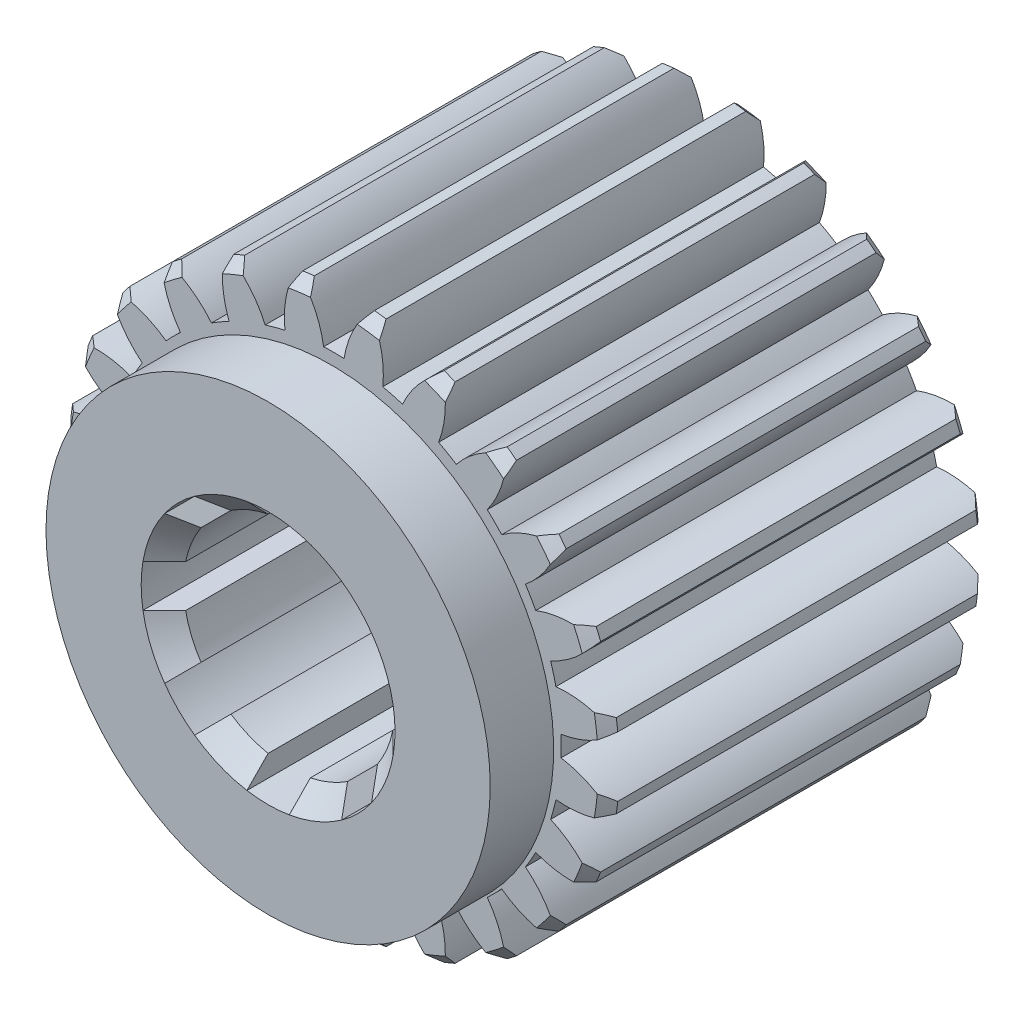
from build123d import *

# Parameters (mm, degrees)
BOSS_EXTRUDE1_DEPTH = 18
SKETCH2_R           = 10.5
BOSS_EXTRUDE2_DEPTH = 3
CUT_EXTRUDE1_DEPTH  = 43.00000000000001
CHAMFER1_SIZE       = 1
CHAMFER2_SIZE       = 0.5
CHAMFER3_SIZE       = 0.5


with BuildPart() as part:
    # Sketch1 → Boss-Extrude1 (new body)
    with BuildSketch(Plane.XY):
        with BuildLine():
            ThreePointArc((-12.813792243846223, 1.7470560088445317), (-11.780957931307613, 1.140113023790045), (-10.629995743569133, 0.8078291893048202))
            ThreePointArc((-10.629995743569133, 0.8078291893048202), (-10.640873065015485, 0.3243808049535287), (-10.629995743569129, -0.15906757939776273))
            ThreePointArc((-10.629995743569129, -0.15906757939776273), (-11.780957931307606, -0.49135141388299797), (-12.813792243846212, -1.0982943989374916))
            ThreePointArc((-12.813792243846212, -1.0982943989374916), (-12.780656262875008, -1.3724596939071496), (-12.741703962830215, -1.6458592559440115))
            ThreePointArc((-12.741703962830215, -1.6458592559440115), (-11.586974222248184, -1.9648039697727557), (-10.389228735284952, -1.9878745727808178))
            ThreePointArc((-10.389228735284952, -1.9878745727808178), (-10.274609771796674, -2.4576651108534753), (-10.13897743689663, -2.9218251330260894))
            ThreePointArc((-10.13897743689663, -2.9218251330260894), (-11.164720154370919, -3.5406776047933204), (-12.005273087305993, -4.3942566996627965))
            ThreePointArc((-12.005273087305993, -4.3942566996627965), (-11.902306987662186, -4.650503815792648), (-11.793920941477731, -4.9045059165580325))
            ThreePointArc((-11.793920941477731, -4.9045059165580325), (-10.595988696391819, -4.91371680399467), (-9.433084285772368, -4.626001952056541))
            ThreePointArc((-9.433084285772368, -4.626001952056541), (-9.200780130294392, -5.050119195046481), (-8.949635901421074, -5.463359116590063))
            ThreePointArc((-8.949635901421074, -5.463359116590063), (-9.78025647755529, -6.326606452390418), (-10.371245737586712, -7.36865165236567))
            ThreePointArc((-10.371245737586712, -7.36865165236567), (-10.2054664888015, -7.589517772159847), (-10.035033026408444, -7.806812588244913))
            ThreePointArc((-10.035033026408444, -7.806812588244913), (-8.875535379644617, -7.505661942532346), (-7.826722059162263, -6.926768927336334))
            ThreePointArc((-7.826722059162263, -6.926768927336334), (-7.492563855989644, -7.276309986020675), (-7.143022797305303, -7.610468189193288))
            ThreePointArc((-7.143022797305303, -7.610468189193288), (-7.721915812501304, -8.659281509675647), (-8.023066458213858, -9.81877915643948))
            ThreePointArc((-8.023066458213858, -9.81877915643948), (-7.8057716421287955, -9.989212618832529), (-7.584905522334614, -10.15499186761774))
            ThreePointArc((-7.584905522334614, -10.15499186761774), (-6.542860322359367, -9.564002607586307), (-5.679612986559018, -8.733382031452082))
            ThreePointArc((-5.679612986559018, -8.733382031452082), (-5.26637306501543, -8.9845262603254), (-4.842255822025492, -9.216830415803367))
            ThreePointArc((-4.842255822025492, -9.216830415803367), (-5.12997067396361, -10.37973482642282), (-5.12075978652696, -11.577667071508737))
            ThreePointArc((-5.12075978652696, -11.577667071508737), (-4.8667576857615735, -11.686053117693186), (-4.610510569631721, -11.789019217336993))
            ThreePointArc((-4.610510569631721, -11.789019217336993), (-3.7569314747622538, -10.948466284401908), (-3.1380790029950347, -9.92272356692761))
            ThreePointArc((-3.1380790029950347, -9.92272356692761), (-2.6739189808224175, -10.058355901827646), (-2.2041284427497603, -10.17297486531592))
            ThreePointArc((-2.2041284427497603, -10.17297486531592), (-2.181057839741687, -11.370720352279156), (-1.8621131259129284, -12.525450092861185))
            ThreePointArc((-1.8621131259129284, -12.525450092861185), (-1.5887135638760694, -12.564402392905972), (-1.314548268906408, -12.597538373877175))
            ThreePointArc((-1.314548268906408, -12.597538373877175), (-0.707605283851926, -11.564704061338563), (-0.3753214493667028, -10.413741873600085))
            ThreePointArc((-0.3753214493667028, -10.413741873600085), (0.10812693498458899, -10.424619195046436), (0.5915753193358801, -10.413741873600078))
            ThreePointArc((0.5915753193358801, -10.413741873600078), (0.9238591538211196, -11.564704061338553), (1.5308021388756163, -12.597538373877157))
            ThreePointArc((1.5308021388756163, -12.597538373877157), (1.8049674338452775, -12.56440239290595), (2.0783669958821362, -12.525450092861156))
            ThreePointArc((2.0783669958821362, -12.525450092861156), (2.397311709710877, -11.370720352279124), (2.420382312718934, -10.17297486531589))
            ThreePointArc((2.420382312718934, -10.17297486531589), (2.890172850791588, -10.058355901827609), (3.3543328729642052, -9.92272356692757))
            ThreePointArc((3.3543328729642052, -9.92272356692757), (3.973185344731441, -10.948466284401857), (4.82676443960092, -11.789019217336927))
            ThreePointArc((4.82676443960092, -11.789019217336927), (5.083011555730775, -11.686053117693115), (5.337013656496155, -11.577667071508664))
            ThreePointArc((5.337013656496155, -11.577667071508664), (5.346224543932788, -10.37973482642275), (5.0585096919946535, -9.216830415803301))
            ThreePointArc((5.0585096919946535, -9.216830415803301), (5.48262693498459, -8.984526260325323), (5.8958668565281735, -8.733382031452003))
            ThreePointArc((5.8958668565281735, -8.733382031452003), (6.759114192328532, -9.564002607586215), (7.801159392303788, -10.154991867617632))
            ThreePointArc((7.801159392303788, -10.154991867617632), (8.022025512097965, -9.98921261883242), (8.239320328183027, -9.818779156439367))
            ThreePointArc((8.239320328183027, -9.818779156439367), (7.9381696824704555, -8.65928150967554), (7.359276667274441, -7.6104681891931865))
            ThreePointArc((7.359276667274441, -7.6104681891931865), (7.70881772595878, -7.276309986020568), (8.04297592913139, -6.926768927336224))
            ThreePointArc((8.04297592913139, -6.926768927336224), (9.091789249613754, -7.505661942532223), (10.25128689637759, -7.806812588244771))
            ThreePointArc((10.25128689637759, -7.806812588244771), (10.421720358770637, -7.589517772159706), (10.587499607555847, -7.368651652365527))
            ThreePointArc((10.587499607555847, -7.368651652365527), (9.99651034752441, -6.32660645239028), (9.16588977139018, -5.463359116589936))
            ThreePointArc((9.16588977139018, -5.463359116589936), (9.417034000263495, -5.050119195046348), (9.649338155741464, -4.6260019520564075))
            ThreePointArc((9.649338155741464, -4.6260019520564075), (10.81224256636092, -4.913716803994523), (12.010174811446836, -4.904505916557867))
            ThreePointArc((12.010174811446836, -4.904505916557867), (12.118560857631284, -4.650503815792484), (12.221526957275088, -4.394256699662628))
            ThreePointArc((12.221526957275088, -4.394256699662628), (11.38097402434, -3.5406776047931636), (10.355231306865702, -2.9218251330259473))
            ThreePointArc((10.355231306865702, -2.9218251330259473), (10.490863641765738, -2.4576651108533283), (10.605482605254009, -1.987874572780672))
            ThreePointArc((10.605482605254009, -1.987874572780672), (11.803228092217243, -1.964803969772595), (12.95795783279927, -1.645859255943833))
            ThreePointArc((12.95795783279927, -1.645859255943833), (12.996910132844057, -1.3724596939069729), (13.030046113815263, -1.0982943989373104))
            ThreePointArc((13.030046113815263, -1.0982943989373104), (11.997211801276649, -0.491351413882831), (10.846249613538166, -0.15906757939761407))
            ThreePointArc((10.846249613538166, -0.15906757939761407), (10.857126934984516, 0.32438080495367744), (10.846249613538157, 0.8078291893049688))
            ThreePointArc((10.846249613538157, 0.8078291893049688), (11.997211801276631, 1.1401130237902128), (13.030046113815231, 1.7470560088447138))
            ThreePointArc((13.030046113815231, 1.7470560088447138), (12.996910132844025, 2.0212213038143743), (12.95795783279923, 2.2946208658512317))
            ThreePointArc((12.95795783279923, 2.2946208658512317), (11.803228092217195, 2.6135655796799697), (10.605482605253961, 2.6366361826880222))
            ThreePointArc((10.605482605253961, 2.6366361826880222), (10.49086364176568, 3.106426720760676), (10.355231306865637, 3.5705867429332923))
            ThreePointArc((10.355231306865637, 3.5705867429332923), (11.38097402433992, 4.189439214700531), (12.221526957274989, 5.043018309570014))
            ThreePointArc((12.221526957274989, 5.043018309570014), (12.118560857631179, 5.299265425699867), (12.010174811446728, 5.553267526465247))
            ThreePointArc((12.010174811446728, 5.553267526465247), (10.812242566360812, 5.562478413901877), (9.649338155741361, 5.274763561963738))
            ThreePointArc((9.649338155741361, 5.274763561963738), (9.417034000263383, 5.698880804953673), (9.16588977139006, 6.112120726497256))
            ThreePointArc((9.16588977139006, 6.112120726497256), (9.99651034752427, 6.975368062297618), (10.587499607555683, 8.017413262272875))
            ThreePointArc((10.587499607555683, 8.017413262272875), (10.421720358770472, 8.23827938206705), (10.251286896377419, 8.455574198152114))
            ThreePointArc((10.251286896377419, 8.455574198152114), (9.091789249613592, 8.154423552439539), (8.042975929131241, 7.5755305372435195))
            ThreePointArc((8.042975929131241, 7.5755305372435195), (7.708817725958623, 7.925071595927856), (7.359276667274276, 8.259229799100469))
            ThreePointArc((7.359276667274276, 8.259229799100469), (7.93816968247027, 9.308043119582834), (8.239320328182815, 10.467540766346668))
            ThreePointArc((8.239320328182815, 10.467540766346668), (8.02202551209775, 10.637974228739715), (7.801159392303569, 10.803753477524921))
            ThreePointArc((7.801159392303569, 10.803753477524921), (6.759114192328328, 10.212764217493483), (5.895866856527984, 9.382143641359253))
            ThreePointArc((5.895866856527984, 9.382143641359253), (5.4826269349843955, 9.633287870232564), (5.0585096919944545, 9.865592025710534))
            ThreePointArc((5.0585096919944545, 9.865592025710534), (5.346224543932564, 11.02849643632999), (5.3370136564959045, 12.226428681415904))
            ThreePointArc((5.3370136564959045, 12.226428681415904), (5.083011555730522, 12.334814727600351), (4.826764439600667, 12.437780827244158))
            ThreePointArc((4.826764439600667, 12.437780827244158), (3.9731853447312053, 11.597227894309066), (3.3543328729639916, 10.571485176834765))
            ThreePointArc((3.3543328729639916, 10.571485176834765), (2.8901728507913713, 10.707117511734797), (2.4203823127187154, 10.821736475223068))
            ThreePointArc((2.4203823127187154, 10.821736475223068), (2.3973117097106336, 12.019481962186303), (2.0783669958818662, 13.174211702768332))
            ThreePointArc((2.0783669958818662, 13.174211702768332), (1.8049674338450972, 13.213164002813105), (1.5308021388755269, 13.246299983784297))
            ThreePointArc((1.5308021388755269, 13.246299983784297), (0.923859153821037, 12.213465671245691), (0.5915753193358065, 11.06250348350721))
            ThreePointArc((0.5915753193358065, 11.06250348350721), (0.10812693498451499, 11.073380804953565), (-0.37532144936677647, 11.06250348350721))
            ThreePointArc((-0.37532144936677647, 11.06250348350721), (-0.7076052838520077, 12.21346567124569), (-1.3145482689064982, 13.246299983784297))
            ThreePointArc((-1.3145482689064982, 13.246299983784297), (-1.5887135638761585, 13.213164002813095), (-1.8621131259130195, 13.1742117027683))
            ThreePointArc((-1.8621131259130195, 13.1742117027683), (-2.1810578397417686, 12.01948196218627), (-2.204128442749832, 10.821736475223036))
            ThreePointArc((-2.204128442749832, 10.821736475223036), (-2.673918980822487, 10.70711751173476), (-3.138079002995105, 10.571485176834718))
            ThreePointArc((-3.138079002995105, 10.571485176834718), (-3.756931474762334, 11.59722789430901), (-4.610510569631806, 12.437780827244088))
            ThreePointArc((-4.610510569631806, 12.437780827244088), (-4.86675768576166, 12.334814727600282), (-5.120759786527043, 12.22642868141583))
            ThreePointArc((-5.120759786527043, 12.22642868141583), (-5.129970673963685, 11.028496436329917), (-4.842255822025558, 9.865592025710464))
            ThreePointArc((-4.842255822025558, 9.865592025710464), (-5.266373065015497, 9.63328787023249), (-5.679612986559079, 9.382143641359173))
            ThreePointArc((-5.679612986559079, 9.382143641359173), (-6.5428603223594335, 10.212764217493394), (-7.584905522334687, 10.803753477524815))
            ThreePointArc((-7.584905522334687, 10.803753477524815), (-7.805771642128869, 10.637974228739601), (-8.023066458213927, 10.467540766346554))
            ThreePointArc((-8.023066458213927, 10.467540766346554), (-7.721915812501365, 9.308043119582724), (-7.143022797305358, 8.25922979910037))
            ThreePointArc((-7.143022797305358, 8.25922979910037), (-7.492563855989698, 7.9250715959277525), (-7.826722059162315, 7.575530537243411))
            ThreePointArc((-7.826722059162315, 7.575530537243411), (-8.875535379644672, 8.154423552439415), (-10.035033026408502, 8.455574198151975))
            ThreePointArc((-10.035033026408502, 8.455574198151975), (-10.205466488801553, 8.23827938206691), (-10.371245737586763, 8.01741326227273))
            ThreePointArc((-10.371245737586763, 8.01741326227273), (-9.780256477555337, 6.9753680622974805), (-8.949635901421113, 6.11212072649713))
            ThreePointArc((-8.949635901421113, 6.11212072649713), (-9.20078013029443, 5.698880804953545), (-9.4330842857724, 5.2747635619636055))
            ThreePointArc((-9.4330842857724, 5.2747635619636055), (-10.595988696391855, 5.5624784139017285), (-11.79392094147777, 5.553267526465081))
            ThreePointArc((-11.79392094147777, 5.553267526465081), (-11.902306987662223, 5.299265425699695), (-12.005273087306028, 5.043018309569842))
            ThreePointArc((-12.005273087306028, 5.043018309569842), (-11.164720154370945, 4.189439214700371), (-10.138977436896651, 3.5705867429331506))
            ThreePointArc((-10.138977436896651, 3.5705867429331506), (-10.274609771796689, 3.106426720760532), (-10.389228735284965, 2.636636182687877))
            ThreePointArc((-10.389228735284965, 2.636636182687877), (-11.586974222248198, 2.6135655796798076), (-12.741703962830229, 2.2946208658510536))
            ThreePointArc((-12.741703962830229, 2.2946208658510536), (-12.780656262875018, 2.021221303814195), (-12.813792243846223, 1.7470560088445317))
        make_face()
    extrude(amount=BOSS_EXTRUDE1_DEPTH)

    # Sketch2 → Boss-Extrude2 (add)
    with BuildSketch(Plane.XY.offset(18)):
        with Locations(Location((0, 0, 0), (0, 0, 207.667206179))):
            Circle(SKETCH2_R)
    extrude(amount=BOSS_EXTRUDE2_DEPTH)

    # Sketch3 → Cut-Extrude1 (cut)
    with BuildSketch(Plane.XY.offset(20.999999999999996)):
        with BuildLine():
            Line((-1, 5.916079783099617), (-1.0000000000000002, 4.898979485566357))
            ThreePointArc((-1.0000000000000002, 4.898979485566357), (-1.9134171618255031, 4.619397662556413), (-2.7569948339513024, 4.171208396324235))
            Line((-2.7569948339513024, 4.171208396324235), (-3.476193351483831, 4.890406913856925))
            ThreePointArc((-3.476193351483831, 4.890406913856925), (-4.242640687119324, 4.242640687119247), (-4.890406913857022, 3.4761933514837633))
            Line((-4.890406913857022, 3.4761933514837633), (-4.171208396324398, 2.75699483395114))
            ThreePointArc((-4.171208396324398, 2.75699483395114), (-4.619397662556495, 1.9134171618254148), (-4.898979485566356, 1))
            Line((-4.898979485566356, 1), (-5.916079783099616, 0.9999999999999996))
            ThreePointArc((-5.916079783099616, 0.9999999999999996), (-6, 7.3e-16), (-5.916079783099617, -1.0000000000000002))
            Line((-5.916079783099617, -1.0000000000000002), (-4.898979485566357, -1.0000000000000002))
            ThreePointArc((-4.898979485566357, -1.0000000000000002), (-4.619397662556435, -1.9134171618254499), (-4.171208396324302, -2.756994833951207))
            Line((-4.171208396324302, -2.756994833951207), (-4.890406913856927, -3.476193351483831))
            ThreePointArc((-4.890406913856927, -3.476193351483831), (-4.242640687119286, -4.2426406871192865), (-3.476193351483831, -4.890406913856926))
            Line((-3.476193351483831, -4.890406913856926), (-2.756994833951207, -4.171208396324302))
            ThreePointArc((-2.756994833951207, -4.171208396324302), (-1.9134171618254485, -4.619397662556434), (-1.0000000000000002, -4.898979485566356))
            Line((-1.0000000000000002, -4.898979485566356), (-1, -5.916079783099616))
            ThreePointArc((-1, -5.916079783099616), (3.7e-16, -6), (0.9999999999999998, -5.916079783099617))
            Line((0.9999999999999998, -5.916079783099617), (1, -4.898979485566357))
            ThreePointArc((1, -4.898979485566357), (1.9134171618254485, -4.619397662556435), (2.7569948339512065, -4.171208396324302))
            Line((2.7569948339512065, -4.171208396324302), (3.47619335148383, -4.890406913856927))
            ThreePointArc((3.47619335148383, -4.890406913856927), (4.242640687119285, -4.2426406871192865), (4.890406913856925, -3.476193351483831))
            Line((4.890406913856925, -3.476193351483831), (4.171208396324301, -2.7569948339512074))
            ThreePointArc((4.171208396324301, -2.7569948339512074), (4.619397662556434, -1.9134171618254492), (4.898979485566356, -1.0000000000000007))
            Line((4.898979485566356, -1.0000000000000007), (5.916079783099616, -1.0000000000000004))
            ThreePointArc((5.916079783099616, -1.0000000000000004), (6, -5e-16), (5.916079783099617, 0.9999999999999996))
            Line((5.916079783099617, 0.9999999999999996), (4.898979485566357, 0.9999999999999996))
            ThreePointArc((4.898979485566357, 0.9999999999999996), (4.619397662556449, 1.9134171618254123), (4.171208396324416, 2.756994833951188))
            Line((4.171208396324416, 2.756994833951188), (4.890406913857039, 3.476193351483811))
            ThreePointArc((4.890406913857039, 3.476193351483811), (4.242640687119409, 4.242640687119277), (3.4761933514839445, 4.890406913856906))
            Line((3.4761933514839445, 4.890406913856906), (2.7569948339513215, 4.171208396324284))
            ThreePointArc((2.7569948339513215, 4.171208396324284), (1.9134171618255156, 4.619397662556458), (1, 4.898979485566357))
            Line((1, 4.898979485566357), (1.0000000000000007, 5.916079783099616))
            ThreePointArc((1.0000000000000007, 5.916079783099616), (3.7e-16, 6), (-1, 5.916079783099617))
        make_face()
    extrude(amount=-CUT_EXTRUDE1_DEPTH, mode=Mode.SUBTRACT)

    # Chamfer1
    chamfer1_edges = [part.edges().sort_by_distance(p)[0] for p in [
        (1.913417161825449, -4.619397662556434, 20.999999999999996),
        (-1.913417161825449, -4.619397662556434, 20.999999999999996),
        (-4.619397662556435, -1.913417161825449, 20.999999999999996),
        (-4.619397662556494, 1.9134171618254174, 20.999999999999996),
        (-1.9134171618255034, 4.619397662556413, 20.999999999999996),
        (1.9134171618255178, 4.619397662556457, 20.999999999999996),
        (4.619397662556448, 1.9134171618254165, 20.999999999999996),
        (4.619397662556434, -1.9134171618254499, 20.999999999999996),
    ]]
    chamfer(chamfer1_edges, length=CHAMFER1_SIZE)

    # Chamfer2
    chamfer2_edges = [part.edges().sort_by_distance(p)[0] for p in [
        (-1.5887135638760697, -12.564402392905968, 18),
        (1.8049674338452775, -12.564402392905947, 18),
        (5.083011555730775, -11.68605311769312, 18),
        (8.022025512097967, -9.989212618832422, 18),
        (10.421720358770635, -7.589517772159704, 18),
        (12.118560857631284, -4.650503815792485, 18),
        (12.996910132844057, -1.3724596939069724, 18),
        (-12.78065626287501, -1.3724596939071532, 18),
        (12.996910132844025, 2.0212213038143743, 18),
        (12.118560857631179, 5.299265425699866, 18),
        (10.421720358770472, 8.238279382067052, 18),
        (8.02202551209775, 10.637974228739719, 18),
        (5.08301155573052, 12.334814727600353, 18),
        (1.804967433845098, 13.213164002813105, 18),
        (-1.5887135638761605, 13.213164002813091, 18),
        (-4.866757685761661, 12.334814727600282, 18),
        (-7.805771642128864, 10.637974228739603, 18),
        (-10.205466488801552, 8.23827938206691, 18),
        (-11.902306987662186, -4.650503815792652, 18),
        (-11.902306987662225, 5.299265425699699, 18),
        (-12.78065626287502, 2.0212213038141944, 18),
        (-10.205466488801497, -7.58951777215985, 18),
        (-7.805771642128793, -9.989212618832532, 18),
        (-4.866757685761575, -11.686053117693184, 18),
    ]]
    chamfer(chamfer2_edges, length=CHAMFER2_SIZE)

    # Chamfer3
    chamfer3_edges = [part.edges().sort_by_distance(p)[0] for p in [
        (8.02202551209775, 10.637974228739719, 0),
        (10.421720358770472, 8.238279382067052, 0),
        (12.118560857631179, 5.299265425699866, 0),
        (12.996910132844025, 2.0212213038143743, 0),
        (12.996910132844057, -1.3724596939069724, 0),
        (12.118560857631284, -4.650503815792485, 0),
        (10.421720358770635, -7.589517772159704, 0),
        (8.022025512097967, -9.989212618832422, 0),
        (5.083011555730775, -11.68605311769312, 0),
        (1.8049674338452775, -12.564402392905947, 0),
        (-1.5887135638760697, -12.564402392905968, 0),
        (-4.866757685761575, -11.686053117693184, 0),
        (-7.805771642128793, -9.989212618832532, 0),
        (-10.205466488801497, -7.58951777215985, 0),
        (-11.902306987662186, -4.650503815792652, 0),
        (-12.78065626287501, -1.3724596939071532, 0),
        (-12.78065626287502, 2.0212213038141944, 0),
        (-11.902306987662225, 5.299265425699699, 0),
        (-10.205466488801552, 8.23827938206691, 0),
        (-7.805771642128864, 10.637974228739603, 0),
        (-4.866757685761661, 12.334814727600282, 0),
        (-1.5887135638761605, 13.213164002813091, 0),
        (1.804967433845098, 13.213164002813105, 0),
        (5.08301155573052, 12.334814727600353, 0),
    ]]
    chamfer(chamfer3_edges, length=CHAMFER3_SIZE)


solid = part.part
